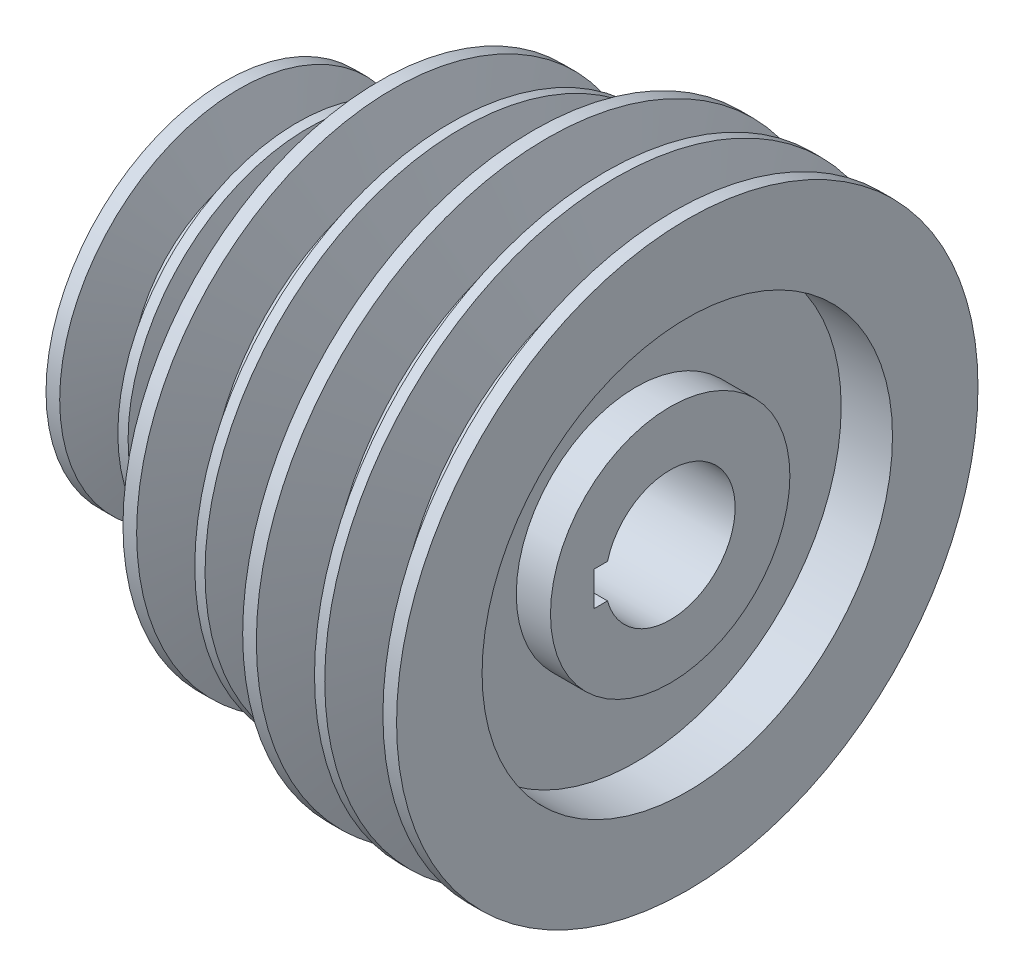
from build123d import *

# Parameters (mm, degrees)
HOLE_WIZARD_M10_1_D     = 8.5
HOLE_WIZARD_M10_1_DEPTH = 24.5
HOLE_WIZARD_M10_1_TIP   = 2.553657631
SKETCH_6_W              = 3.96969722
SKETCH_6_H              = 10
CUT_EXTRUDE_1_DEPTH     = 178.059312096


with BuildPart() as part:
    # 草图1 → 旋转1 (revolve)
    with BuildSketch(Plane.XY, mode=Mode.PRIVATE) as revolve_1_sk:
        Polygon((0, 26), (0, 52.5), (4, 52.5), (8.891690903, 36.5), (16.108309097, 36.5), (21, 52.5), (24, 52.5), (28.891690903, 36.5), (36.108309097, 36.5), (41, 52.5), (45, 52.5), (45, 75), (49, 75), (53.891690903, 59), (61.108309097, 59), (66, 75), (69, 75), (73.891690903, 59), (81.108309097, 59), (86, 75), (90, 75), (90, 85), (94, 85), (98.891690903, 69), (106.108309097, 69), (111, 85), (114, 85), (118.891690903, 69), (126.108309097, 69), (131, 85), (135, 85), (135, 60), (120, 60), (120, 35), (130, 35), (130, 19), (30, 19), (30, 26), align=None)
    revolve(revolve_1_sk.sketch.rotate(Axis((-46.234880066, 0, 0), (1, 0, 0)), 90), axis=Axis((-46.234880066, 0, 0), (1, 0, 0)))

    # M10 螺纹孔1
    with Locations(Plane.ZY):
        with Locations((0, 32), (0, -32)):
            Hole(HOLE_WIZARD_M10_1_D / 2, depth=HOLE_WIZARD_M10_1_DEPTH)
            with Locations((0, 0, -(HOLE_WIZARD_M10_1_DEPTH + HOLE_WIZARD_M10_1_TIP / 2))):  # 118° drill point
                Cone(0, HOLE_WIZARD_M10_1_D / 2, HOLE_WIZARD_M10_1_TIP, mode=Mode.SUBTRACT)

    # 草图6 → 切除-拉伸1 (cut, through all)
    with BuildSketch(Plane(origin=(130, 0, 0), x_dir=(0, 0, -1), z_dir=(1, 0, 0))):
        with Locations((-20.31515139, 0)):
            Rectangle(SKETCH_6_W, SKETCH_6_H)
    extrude(amount=-CUT_EXTRUDE_1_DEPTH, mode=Mode.SUBTRACT)


solid = part.part
